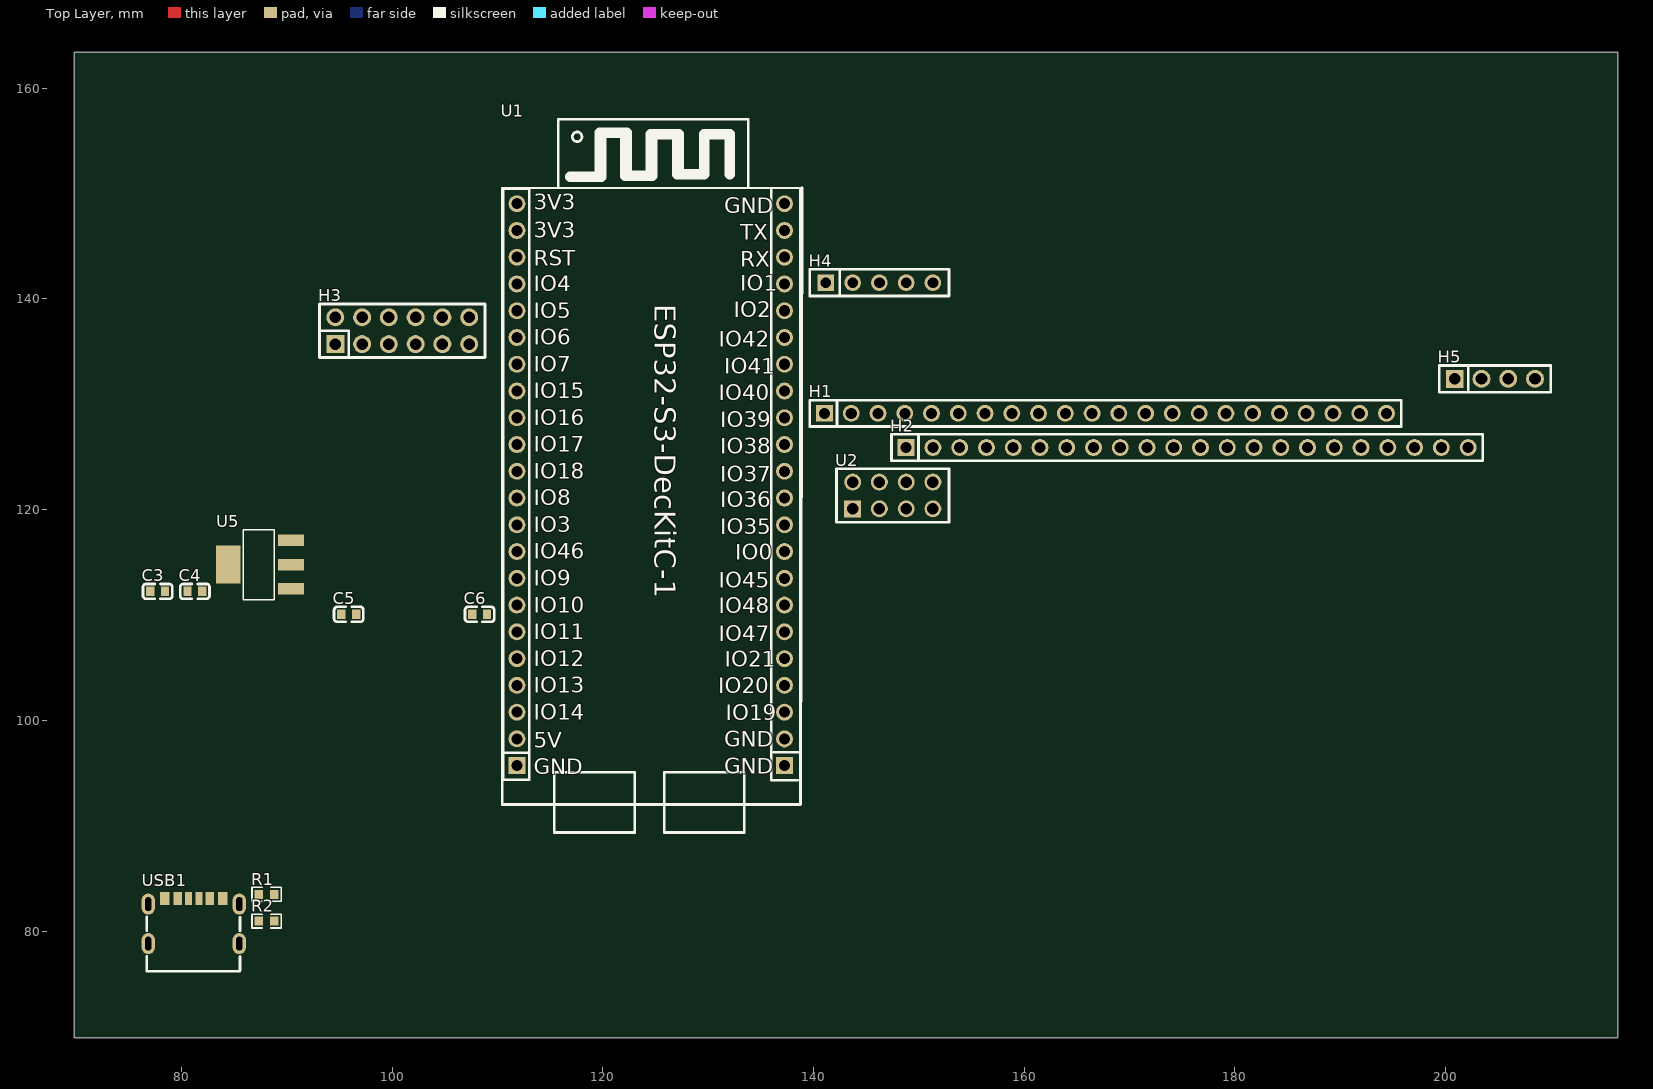
[diagram p0: Top Layer view]
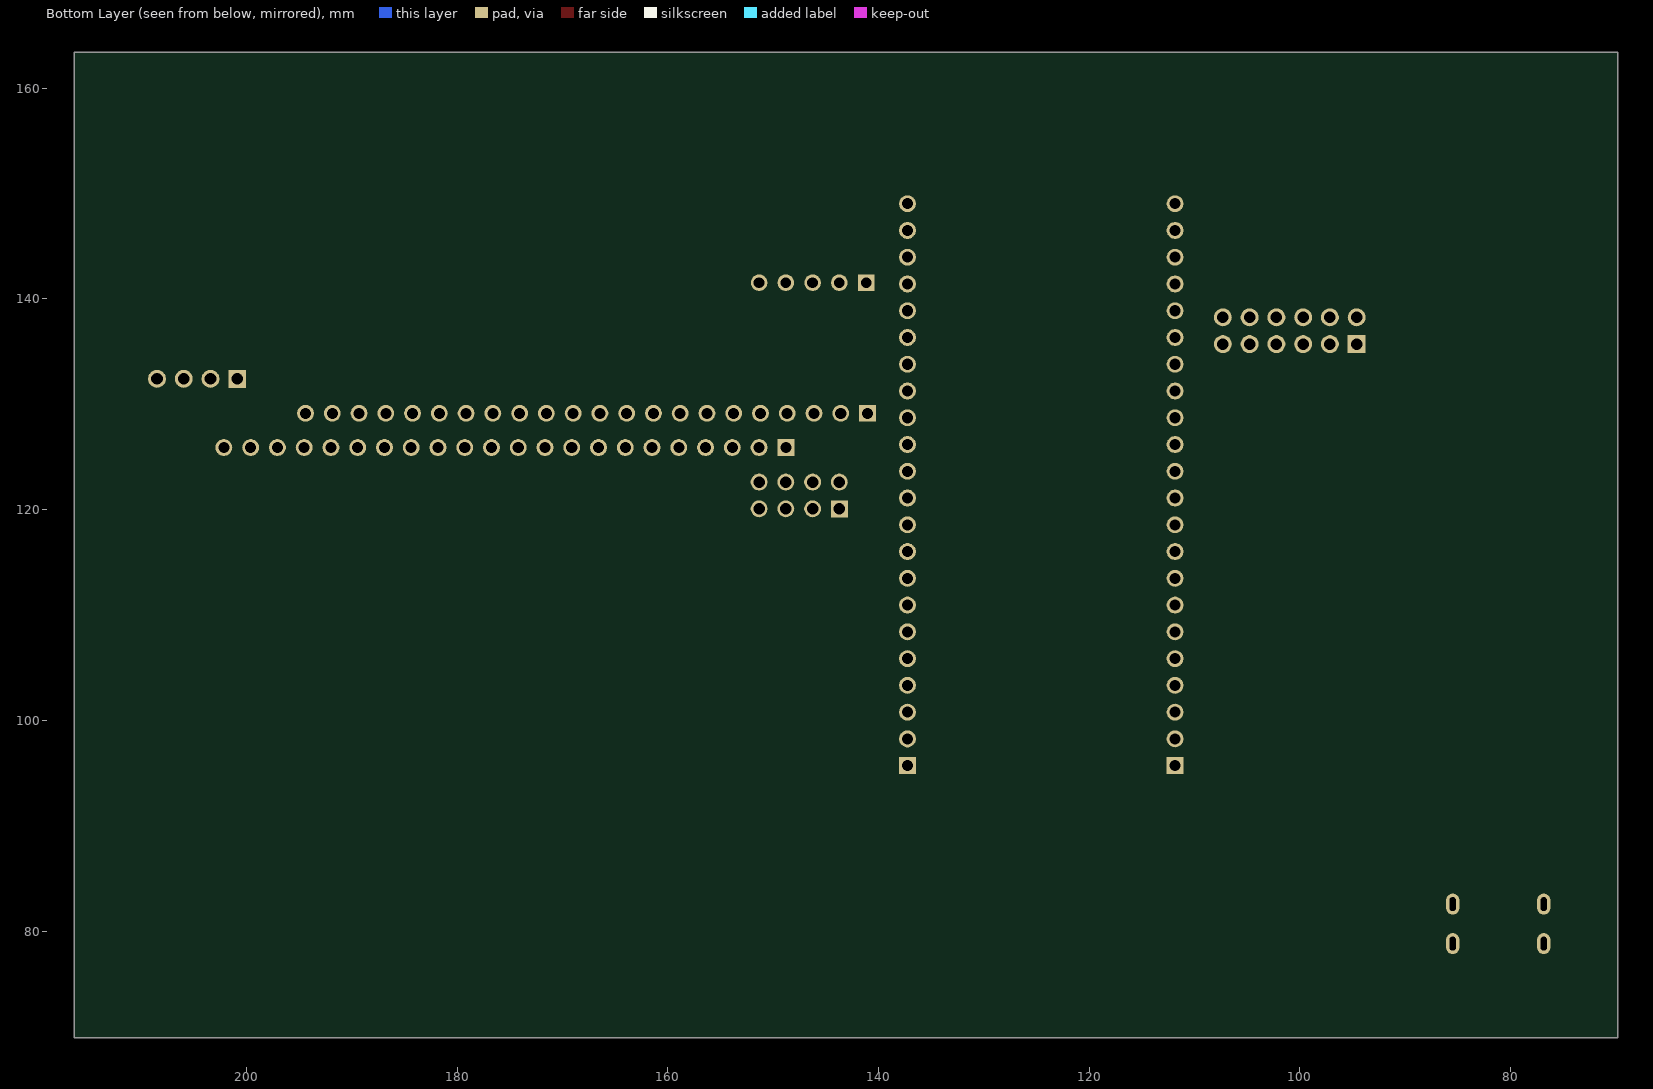
[diagram p1: Bottom Layer view, seen from below]
# Altium PCB MISC49904.pcbdoc
Units mm, origin at the board's own origin, x right, y up, seen from the top; angles counter-clockwise.
Board outline 146.46 x 93.54 mm, 2 copper layers (Top Layer, Bottom Layer), stack 1.58 mm thick; 15 components, 25 nets, 143 pads, 0 vias.

## Layer stack, top to bottom
Top Solder Mask Layer: solder mask 0.01, Dk 3.3
Top Layer: signal copper 0.035
Dielectric1: surface 1.51, FR4, Dk 4.5
Bottom Layer: signal copper 0.035
Bottom Solder Mask Layer: solder mask 0.01, Dk 3.3

## Board outline
216.309,69.85 69.85,69.85 69.85,163.391 216.309,163.391

## Design rules (kind name [scope] priority, off if disabled: settings)
BoardOutlineClearance copperThickness2oz_1 [All] p2 off: genericclearance=0.203 ignorepadtopadclearanceinfootprint=FALSE except(0: Arc-SplitContinuation Track-SplitContinuation SMDPad-SplitContinuation THPad-SplitContinuation Via-SplitContinuation Fill-SplitContinuation Region-SplitContinuation Poly-SplitContinuation Text-SplitContinuation Hole-SplitContinuation; 0.152: Arc-CutoutEdge SMDPad-CutoutEdge THPad-CutoutEdge Via-CutoutEdge Fill-CutoutEdge Region-CutoutEdge Text-CutoutEdge; 0.176: Hole-OutlineEdge Hole-CutoutEdge; 0.254: Poly-OutlineEdge Poly-CutoutEdge; 0.3: Arc-OutlineEdge Track-OutlineEdge SMDPad-OutlineEdge THPad-OutlineEdge Via-OutlineEdge Fill-OutlineEdge Region-OutlineEdge Text-OutlineEdge Track-CutoutEdge)
BoardOutlineClearance copperThickness1oz_1 [All] p4: genericclearance=0.102 ignorepadtopadclearanceinfootprint=FALSE except(0: Arc-SplitContinuation Track-SplitContinuation SMDPad-SplitContinuation THPad-SplitContinuation Via-SplitContinuation Fill-SplitContinuation Region-SplitContinuation Poly-SplitContinuation Text-SplitContinuation Hole-SplitContinuation; 0.152: SMDPad-CutoutEdge THPad-CutoutEdge Via-CutoutEdge Fill-CutoutEdge Region-CutoutEdge Text-CutoutEdge; 0.176: Hole-OutlineEdge Hole-CutoutEdge; 0.254: Poly-OutlineEdge Poly-CutoutEdge; 0.3: Arc-OutlineEdge Track-OutlineEdge SMDPad-OutlineEdge THPad-OutlineEdge Via-OutlineEdge Fill-OutlineEdge Region-OutlineEdge Text-OutlineEdge Arc-CutoutEdge Track-CutoutEdge)
Clearance copperThickness2oz [All] p1 off: gap=0.203 ignorepadtopadclearanceinfootprint=FALSE except(0.152: SMDPad-Track SMDPad-SMDPad THPad-Track SMDPad-THPad THPad-THPad Track-Via SMDPad-Via THPad-Via Via-Via Fill-Track Region-Track Fill-SMDPad Region-SMDPad Fill-THPad Region-THPad Fill-Via Region-Via Fill-Fill Fill-Region Region-Region Arc-Track Arc-SMDPad Arc-THPad Arc-Via Fill-Arc Region-Arc Arc-Arc Text-Track SMDPad-Text Text-THPad Text-Via Fill-Text Region-Text Arc-Text Text-Text; 0.176: Hole-Track Hole-SMDPad Hole-THPad Hole-Via Fill-Hole Region-Hole Hole-Arc Hole-Text; 0.254: Poly-Track Poly-SMDPad Poly-THPad Poly-Via Poly-Fill Poly-Region Poly-Poly Poly-Arc Poly-Text Poly-Hole)
Clearance copperThickness1oz [All] p3: gap=0.102 ignorepadtopadclearanceinfootprint=FALSE except(0.152: SMDPad-Track SMDPad-SMDPad THPad-Track SMDPad-THPad THPad-THPad Track-Via SMDPad-Via THPad-Via Via-Via Fill-Track Region-Track Fill-SMDPad Region-SMDPad Fill-THPad Region-THPad Fill-Via Region-Via Fill-Fill Fill-Region Region-Region Arc-Track Arc-SMDPad Arc-THPad Arc-Via Fill-Arc Region-Arc Arc-Arc Text-Track SMDPad-Text Text-THPad Text-Via Fill-Text Region-Text Arc-Text Text-Text; 0.176: Hole-Track Hole-SMDPad Hole-THPad Hole-Via Fill-Hole Region-Hole Hole-Arc Hole-Text; 0.254: Poly-Track Poly-SMDPad Poly-THPad Poly-Via Poly-Fill Poly-Region Poly-Poly Poly-Arc Poly-Text Poly-Hole)
DiffPairsRouting differentialPair [All] p1: maxlimit=0.152 minlimit=0.152 mostfreqgap=0.152 toplayer_minwidth=0.127 toplayer_prefwidth=0.254 toplayer_maxwidth=2.54 toplayer_mingap=0.152 toplayer_prefgap=0.152 toplayer_maxgap=0.152 bottomlayer_minwidth=0.127 bottomlayer_prefwidth=0.254 bottomlayer_maxwidth=2.54 bottomlayer_mingap=0.152 bottomlayer_prefgap=0.152 bottomlayer_maxgap=0.152 maxuncoupledlength=0.254
HoleToHoleClearance otherClearance [All] p1: gap=0.3 allowstackedmicrovias=TRUE
Length netLength [All] p1: minlimit=0 maxlimit=0
MatchedLengths netLengthTolerance [All] p1: tolerance=25.4
PasteMaskExpansion pasteMaskExpansion [All] p1: expansion=0
PlaneConnect innerPlane [All] p1: planeconnectstyle=Relief reliefexpansion=0.508 reliefentries=4 reliefconductorwidth=0.254 reliefairgap=0.254
PolygonConnect copperRegion [All] p1: connectstyle=Relief reliefconductorwidth=0.254 reliefentries=4 polygonreliefangle="90 Angle" airgapwidth=0.254 via.connectstyle=Relief via.reliefconductorwidth=0.254 via.reliefentries=4 via.polygonreliefangle="90 Angle" via.airgapwidth=0.254
RoutingVias viaSize [All] p1: holewidth=0.305 width=0.61 viastyle="Through Hole" minholewidth=0.3 minwidth=0.5 maxholewidth=6.3 maxwidth=10
SolderMaskExpansion solderMaskExpansion [IsVia] p1: expansion=-25.4 istentingtop=TRUE
SolderMaskExpansion solderMaskExpansion [All] p2: expansion=0.051 istentingtop=FALSE
Width copperThickness2oz_2 [All] p1 off: maxlimit=2.54 minlimit=0.203 preferedwidth=0.254
Width copperThickness1oz_2 [All] p2: maxlimit=2.54 minlimit=0.127 preferedwidth=0.254

## Components (designator, comment, footprint, x,y, rotation, side; value= is the part's Value field where it differs from the comment)
C3 "10uF" C0603 77.739,112.238 r0 top
C4 "100nF" C0603 81.273,112.238 r0 top
C5 "10uF" C0603 95.879,110.063 r0 top
C6 "100nF" C0603 108.303,110.063 r0 top
H1 "CS-1165SDIG-1*22" HDR-TH_22P-P2.54-V-F 167.709,129.145 r0 top
H2 "CS-1165SDIG-1*22" HDR-TH_22P-P2.54-V-F 175.459,125.891 r0 top
H3 "LD3320" HDR-TH_12P-P2.54-V-F-R2-C6-S2.54 100.959,136.983 r0 top
H4 "SYN6288" HDR-TH_5P-P2.54-V-F 146.249,141.547 r0 top
H5 "OLED" HDR-TH_4P-P2.54-V-F 204.669,132.419 r0 top
R1 "5.1K" R0603 88.079,83.486 r0 top
R2 "5.1K" R0603 88.079,80.946 r0 top
U1 "ESP32-S3-DEVKITC-1-1000MIL" ESP32-S3-DEVKITC-1-1000MIL 116.797,122.497 r0 top
U2 "max30102" HDR-TH_8P-P2.54-V-F-R2-C4-S2.54 147.519,121.347 r0 top
U5 "AMS1117-3.3" SOT-223-3_L6.5-W3.4-P2.30-LS7.0-BR 87.43,114.778 r0 top
USB1 "" "USB_ TYPE-C-6P" 81.043,80.946 r0 top

## Footprints (in the part's own frame and the unit in brackets; to place one, negate y for a bottom-side part, rotate by r counter-clockwise, add the part's x,y. Pads: shape width x height; smd on the part's side, far side on the other; paste and mask are expansions set on the pad)
C0603 [mm]
  rect 0.8x0.9 smd: 1(-0.7,0) 2(0.7,0)
  silkscreen extent -1.39,-0.71 1.39,0.71
ESP32-S3-DEVKITC-1-1000MIL [mm]
  round 1.6 hole 1.05 paste+0 mask+0.051: 1(-4.953,26.543) 2(-4.953,24.003) 3(-4.953,21.463) 4(-4.953,18.923) 5(-4.953,16.383) 6(-4.953,13.843) 7(-4.953,11.303) 8(-4.953,8.763) 9(-4.953,6.223) 10(-4.953,3.683) 11(-4.953,1.143) 12(-4.953,-1.397) 13(-4.953,-3.937) 14(-4.953,-6.477) 15(-4.953,-9.017) 16(-4.953,-11.557) 17(-4.953,-14.097) 18(-4.953,-16.637) 19(-4.953,-19.177) 20(-4.953,-21.717) 21(-4.953,-24.257)
  rect 1.6x1.6 hole 1.05 paste+0 mask+0.051: 22(-4.953,-26.797) 44(20.447,-26.797)
  round 1.6 hole 1.05 copper offset 0,0 paste+0 mask+0.051: 23(20.447,26.543) 24(20.447,24.003) 25(20.447,21.463) 26(20.447,18.923) 27(20.447,16.383) 28(20.447,13.843) 29(20.447,11.303) 30(20.447,8.763) 31(20.447,6.223) 32(20.447,3.683) 33(20.447,1.143) 34(20.447,-1.397) 35(20.447,-3.937) 36(20.447,-6.477) 37(20.447,-9.017) 38(20.447,-11.557) 39(20.447,-14.097) 40(20.447,-16.637) 41(20.447,-19.177) 42(20.447,-21.717) 43(20.447,-24.257)
  Top Layer circle w0.425: c20.447,26.543 r0.213
  Top Layer circle w0.425: c20.447,24.003 r0.213
  Top Layer circle w0.425: c20.447,21.463 r0.213
  Top Layer circle w0.425: c20.447,18.923 r0.213
  Top Layer circle w0.425: c20.447,16.383 r0.213
  Top Layer circle w0.425: c20.447,13.843 r0.213
  Top Layer circle w0.425: c20.447,11.303 r0.213
  Top Layer circle w0.425: c20.447,8.763 r0.213
  Top Layer circle w0.425: c20.447,6.223 r0.213
  Top Layer circle w0.425: c20.447,3.683 r0.213
  Top Layer circle w0.425: c20.447,1.143 r0.213
  Top Layer circle w0.425: c20.447,-1.397 r0.213
  Top Layer circle w0.425: c20.447,-3.937 r0.213
  Top Layer circle w0.425: c20.447,-6.477 r0.213
  Top Layer circle w0.425: c20.447,-9.017 r0.213
  Top Layer circle w0.425: c20.447,-11.557 r0.213
  Top Layer circle w0.425: c20.447,-14.097 r0.213
  Top Layer circle w0.425: c20.447,-16.637 r0.213
  Top Layer circle w0.425: c20.447,-19.177 r0.213
  Top Layer circle w0.425: c20.447,-21.717 r0.213
  Top Layer circle w0.425: c20.447,-24.257 r0.213
  Top Layer circle w0.425: c20.447,-26.797 r0.213
  Top Layer circle w0.425: c-4.953,26.543 r0.213
  Top Layer circle w0.425: c-4.953,24.003 r0.213
  Top Layer circle w0.425: c-4.953,21.463 r0.213
  Top Layer circle w0.425: c-4.953,18.923 r0.213
  Top Layer circle w0.425: c-4.953,16.383 r0.213
  Top Layer circle w0.425: c-4.953,13.843 r0.213
  Top Layer circle w0.425: c-4.953,11.303 r0.213
  Top Layer circle w0.425: c-4.953,8.763 r0.213
  Top Layer circle w0.425: c-4.953,6.223 r0.213
  Top Layer circle w0.425: c-4.953,3.683 r0.213
  Top Layer circle w0.425: c-4.953,1.143 r0.213
  Top Layer circle w0.425: c-4.953,-1.397 r0.213
  Top Layer circle w0.425: c-4.953,-3.937 r0.213
  Top Layer circle w0.425: c-4.953,-6.477 r0.213
  Top Layer circle w0.425: c-4.953,-9.017 r0.213
  Top Layer circle w0.425: c-4.953,-11.557 r0.213
  Top Layer circle w0.425: c-4.953,-14.097 r0.213
  Top Layer circle w0.425: c-4.953,-16.637 r0.213
  Top Layer circle w0.425: c-4.953,-19.177 r0.213
  Top Layer circle w0.425: c-4.953,-21.717 r0.213
  Top Layer circle w0.425: c-4.953,-24.257 r0.213
  Top Layer circle w0.425: c-4.953,-26.797 r0.213
  silkscreen extent -6.35,-33.15 22.1,34.54
HDR-TH_4P-P2.54-V-F [mm]
  rect 1.7x1.7 hole 1.1: 1(-3.81,0)
  round 1.7 hole 1.1: 2(-1.27,0) 3(1.27,0) 4(3.81,0)
  silkscreen extent -5.29,-1.27 5.29,1.27
HDR-TH_5P-P2.54-V-F [mil]
  rect 62x62 hole 40.16: 1(-200,0)
  round 62 hole 40.16: 2(-100,0) 3(0,0) 4(100,0) 5(200,0)
  silkscreen extent -260,-50 260,50
HDR-TH_8P-P2.54-V-F-R2-C4-S2.54 [mm]
  rect 1.6x1.6 hole 1.1: 1(-3.81,-1.27)
  round 1.6 hole 1.1: 2(-3.81,1.27) 3(-1.27,-1.27) 4(-1.27,1.27) 5(1.27,-1.27) 6(1.27,1.27) 7(3.81,-1.27) 8(3.81,1.27)
  silkscreen extent -5.33,-2.54 5.33,2.54
HDR-TH_12P-P2.54-V-F-R2-C6-S2.54 [mm]
  rect 1.7x1.7 hole 1.1: 1(-6.35,-1.27)
  round 1.7 hole 1.1: 2(-6.35,1.27) 3(-3.81,-1.27) 4(-3.81,1.27) 5(-1.27,-1.27) 6(-1.27,1.27) 7(1.27,-1.27) 8(1.27,1.27) 9(3.81,-1.27) 10(3.81,1.27) 11(6.35,-1.27) 12(6.35,1.27)
  silkscreen extent -7.85,-2.54 7.85,2.54
HDR-TH_22P-P2.54-V-F [mm]
  rect 1.6x1.6 hole 1.05: 1(-26.67,0)
  round 1.6 hole 1.05: 2(-24.13,0) 3(-21.59,0) 4(-19.05,0) 5(-16.51,0) 6(-13.97,0) 7(-11.43,0) 8(-8.89,0) 9(-6.35,0) 10(-3.81,0) 11(-1.27,0) 12(1.27,0) 13(3.81,0) 14(6.35,0) 15(8.89,0) 16(11.43,0) 17(13.97,0) 18(16.51,0) 19(19.05,0) 20(21.59,0) 21(24.13,0) 22(26.67,0)
  silkscreen extent -28.06,-1.25 28.06,1.25
R0603 [mm]
  rect 0.806x0.864 smd paste-100 mask+0.051: 1(-0.753,0) 2(0.753,0)
  silkscreen extent -1.39,-0.66 1.39,0.66
SOT-223-3_L6.5-W3.4-P2.30-LS7.0-BR [mm]
  rect 2.5x1.1 smd: 1(2.97,-2.3) 2(2.97,0) 3(2.97,2.3)
  rect 2.34x3.6 smd: 4(-2.97,0)
  silkscreen extent -1.57,-3.33 1.37,3.33
"USB_ TYPE-C-6P" [mm]
  oval 1.25x2 hole 0.6 slot 1.3 at 90 deg paste+0 mask+0.05: 7(-4.193,1.611) 8(4.447,1.611) 9(-4.193,-2.139) 10(4.447,-2.139)
  rect 0.7x1.2 smd paste-100 mask+0.05: A5(-0.373,2.139) B5(0.627,2.139)
  rect 0.8x1.2 smd paste-100 mask+0.05: A9(1.647,2.139) B9(-1.393,2.139)
  rect 0.9x1.2 smd paste-100 mask+0.05: A12(2.877,2.139) B12(-2.623,2.139)
  silkscreen extent -4.34,-4.75 4.52,0.39

## Nets (pads, with @x,y where several pads share a name; then routed paths per layer and width w, separated by ;. In a path a pad name is that pad's centre, name@x,y a point inside that pad or via, vN(x,y) a via of type N, cw(c..) or ccw(c..) an arc to the next point about the centre after c; other vN are vias at no path point)
3.3v: C5.2 C6.2 U5.2 U5.4
3V3: H1.1 H1.2
5V: H1.21
$1N34: R1.1 USB1.A5
$1N35: R2.1 USB1.B5
+5V: C3.2 C4.2 U5.3 USB1.A9 USB1.B9
GND: C3.1 C4.1 C5.1 C6.1 H1.22 R1.2 R2.2 U5.1 USB1.7 USB1.8 USB1.9 USB1.10 USB1.A12 USB1.B12
IO3: H1.13
IO4: H1.4
IO5: H1.5
IO6: H1.6
IO7: H1.7
IO8: H1.12
IO9: H1.15
IO10: H1.16
IO11: H1.17
IO12: H1.18
IO13: H1.19
IO14: H1.20
IO15: H1.8
IO16: H1.9
IO17: H1.10
IO18: H1.11
IO46: H1.14
RST: H1.3
pads on no net: H2.1 H2.2 H2.3 H2.4 H2.5 H2.6 H2.7 H2.8 H2.9 H2.10 H2.11 H2.12 H2.13 H2.14 H2.15 H2.16 H2.17 H2.18 H2.19 H2.20 H2.21 H2.22 H3.1 H3.2 H3.3 H3.4 H3.5 H3.6 H3.7 H3.8 H3.9 H3.10 H3.11 H3.12 H4.1 H4.2 H4.3 H4.4 H4.5 H5.1 H5.2 H5.3 H5.4 U1.1 U1.2 U1.3 U1.4 U1.5 U1.6 U1.7 U1.8 U1.9 U1.10 U1.11 U1.12 U1.13 U1.14 U1.15 U1.16 U1.17 U1.18 U1.19 U1.20 U1.21 U1.22 U1.23 U1.24 U1.25 U1.26 U1.27 U1.28 U1.29 U1.30 U1.31 U1.32 U1.33 U1.34 U1.35 U1.36 U1.37 U1.38 U1.39 U1.40 U1.41 U1.42 U1.43 U1.44 U2.1 U2.2 U2.3 U2.4 U2.5 U2.6 U2.7 U2.8